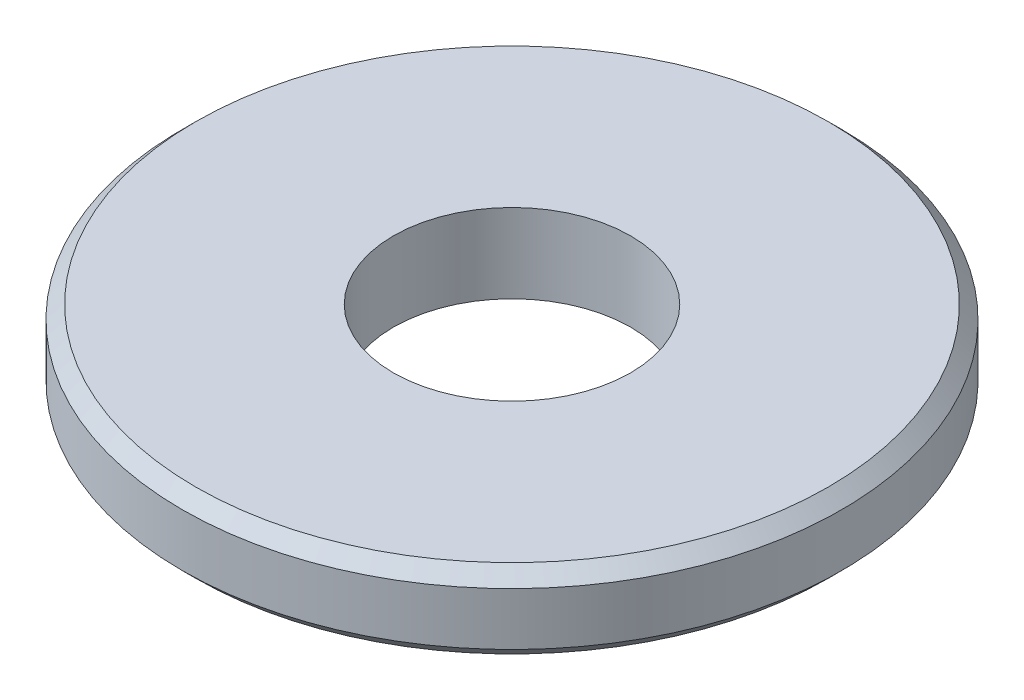
SolidWorks part; units mm, degrees
ref_plane "前视基准面" through (0, 0, 0) normal (0, 0, 1) x (1, 0, 0)
ref_plane "上视基准面" through (0, 0, 0) normal (0, 1, 0) x (1, 0, 0)
ref_plane "右视基准面" through (0, 0, 0) normal (1, 0, 0) x (0, 0, -1)
sketch "草图1" plane through (0, 0, 0) normal (0, 1, 0) x (1, 0, 0)
  circle A0 centre (0, 0) radius 12.5
  dimension "D1" = 25
extrude "凸台-拉伸1" add sketch "草图1" along normal blind 3
sketch "草图2" plane through (0, 3, 0) normal (0, 1, 0) x (1, 0, 0)
  circle A0 centre (0, 0) radius 4.5
  dimension "D1" = 9
extrude "切除-拉伸1" cut sketch "草图2" against normal through all
chamfer "倒角1" distance 0.5 angle 45 2 edges at (0, 0, 12.5) (0, 3, 12.5)
